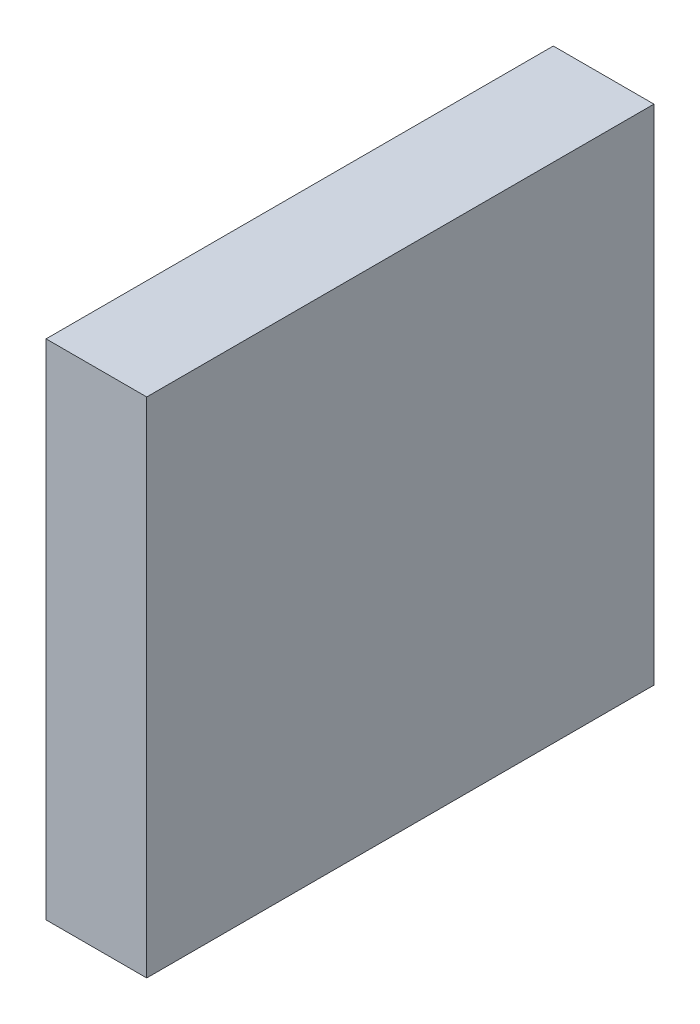
from build123d import *

# Parameters (mm, degrees)
SKETCH2_W           = 25
SKETCH2_H           = 126
BOSS_EXTRUDE1_DEPTH = 62.5


with BuildPart() as part:
    # Sketch2 → Boss-Extrude1 (new, symmetric)
    with BuildSketch(Plane(origin=(0, 0, 0), x_dir=(1, 0, 0), z_dir=(0, 1, 0))):
        Rectangle(SKETCH2_W, SKETCH2_H)
    extrude(amount=BOSS_EXTRUDE1_DEPTH, both=True)


solid = part.part
